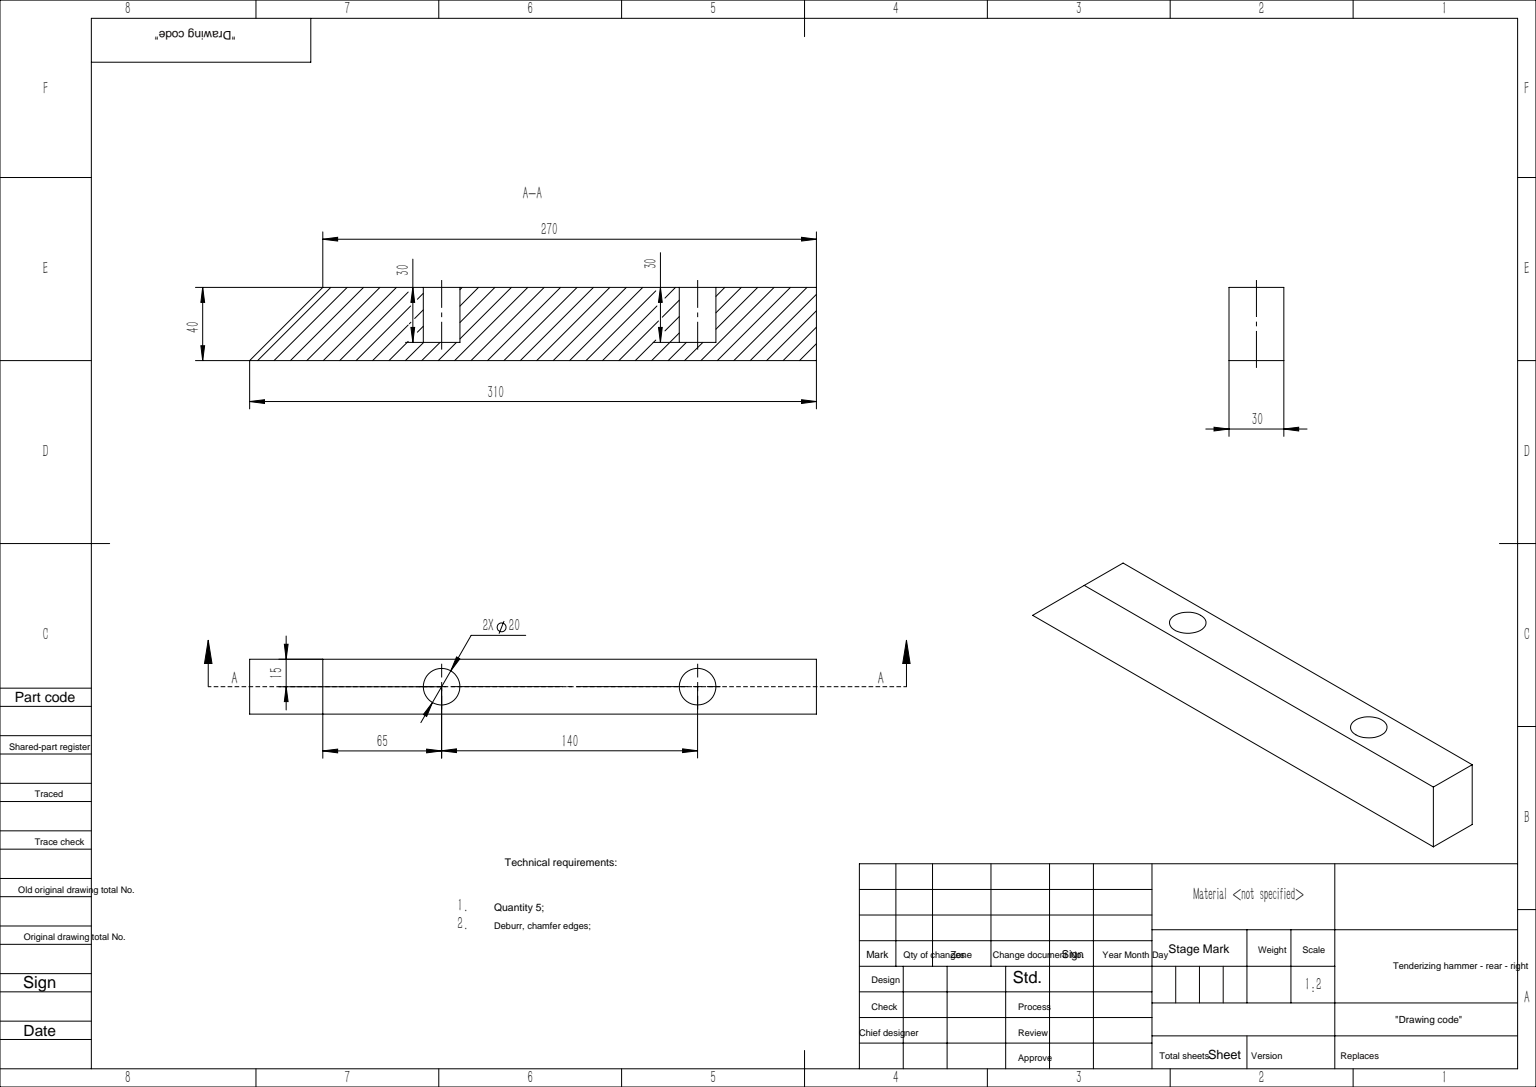
SolidWorks part; units mm, degrees
ref_plane "前视基准面" through (0, 0, 0) normal (0, 0, 1) x (1, 0, 0)
ref_plane "上视基准面" through (0, 0, 0) normal (0, 1, 0) x (1, 0, 0)
ref_plane "右视基准面" through (0, 0, 0) normal (1, 0, 0) x (0, 0, -1)
sketch "草图1" plane through (0, 0, 0) normal (0, 1, 0) x (1, 0, 0)
  line L1 (-135, -15) -> (135, -15)
  line L2 (-135, -15) -> (-135, 15)
  line L3 (-135, 15) -> (135, 15)
  line L4 (135, -15) -> (135, 15)
  line L5 (-135, -15) -> (135, 15) construction
  line L6 (-135, 15) -> (135, -15) construction
  point P0 (0, 0)
  dimension "D1" = 270
  dimension "D2" = 30
extrude "凸台-拉伸1" add sketch "草图1" along normal blind 40
sketch "草图2" plane through (0, 40, 0) normal (0, 1, 0) x (1, 0, 0)
  line L1 (0, 0) -> (0, 40) construction
  circle A0 centre (70, 0) radius 10
  circle A1 centre (-70, 0) radius 10
  dimension "D1" = 20
  dimension "D2" = 140
  dimension "D3" = 40
extrude "切除-拉伸2" cut sketch "草图2" against normal blind 30
sketch "草图3" plane through (-135, 0, 0) normal (-1, 0, 0) x (0, 0, 1)
  line L4 (-15, 0) -> (15, 0)
  line L5 (15, 0) -> (15, 40)
  line L6 (15, 40) -> (-15, 40)
  line L7 (-15, 40) -> (-15, 0)
  line L8 (-15, 0) -> (15, 0)
  line L9 (15, 0) -> (15, 40)
  line L10 (15, 40) -> (-15, 40)
  line L11 (-15, 40) -> (-15, 0)
  dimension "D1" = 0
extrude "凸台-拉伸2" add sketch "草图3" along normal blind 40
sketch "草图4" plane through (0, 0, 15) normal (0, 0, 1) x (1, 0, 0)
  line L0 (-175, 0) -> (-135, 40)
  line L1 (-175, 40) -> (135, 40) construction
  line L2 (-175, 0) -> (-175, 40) construction
  line L3 (-175, 0) -> (-175, 40)
  line L4 (-175, 40) -> (-135, 40)
  dimension "D1" = 45
extrude "切除-拉伸3" cut sketch "草图4" against normal through all
